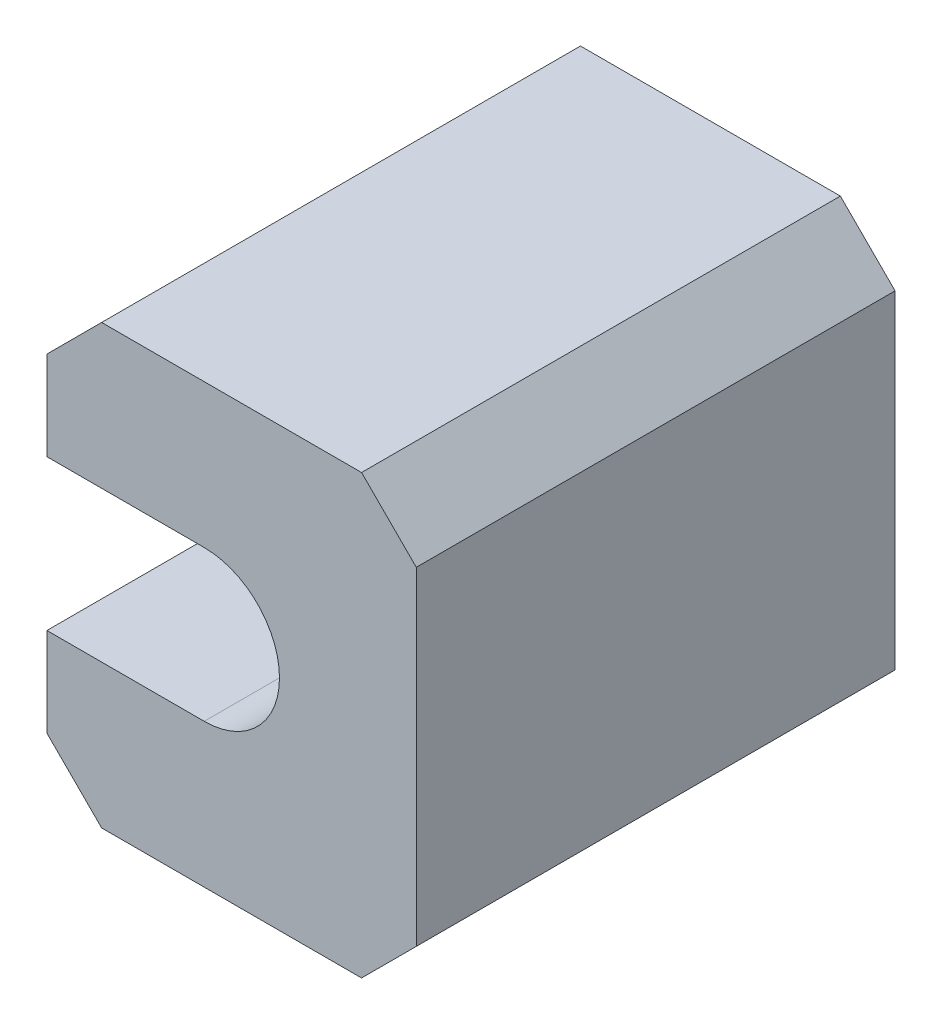
SolidWorks part; units mm, degrees
ref_plane "Front Plane" through (0, 0, 0) normal (0, 0, 1) x (1, 0, 0)
ref_plane "Top Plane" through (0, 0, 0) normal (0, 1, 0) x (1, 0, 0)
ref_plane "Right Plane" through (0, 0, 0) normal (1, 0, 0) x (0, 0, -1)
sketch "Sketch1" plane through (0, 0, 0) normal (0, 0, 1) x (1, 0, 0)
  line L0 (0, 8) -> (0, 56)
  line L1 (-8, 64) -> (-46, 64)
  line L2 (-54, 56) -> (-54, 43)
  line L3 (-54, 43) -> (-31, 43)
  line L4 (-8, 0) -> (-46, 0)
  line L5 (-54, 8) -> (-54, 21)
  line L6 (-54, 21) -> (-31, 21)
  line L7 (-46, 64) -> (-54, 56)
  line L8 (0, 56) -> (-8, 64)
  line L9 (-46, 0) -> (-54, 8)
  line L10 (0, 8) -> (-8, 0)
  arc A0 (-31, 21) -> (-31, 43) centre (-31, 32) ccw
  point P0 (0, 0)
  point P1 (0, 64)
  point P4 (-54, 64)
  point P7 (-54, 0)
  dimension "D4" = 22
  dimension "D1" = 64
  dimension "D2" = 54
  dimension "D3" = 54
  dimension "D5" = 21
  dimension "D6" = 21
  dimension "D7" = 31
extrude "Boss-Extrude1" add sketch "Sketch1" along normal blind 70
